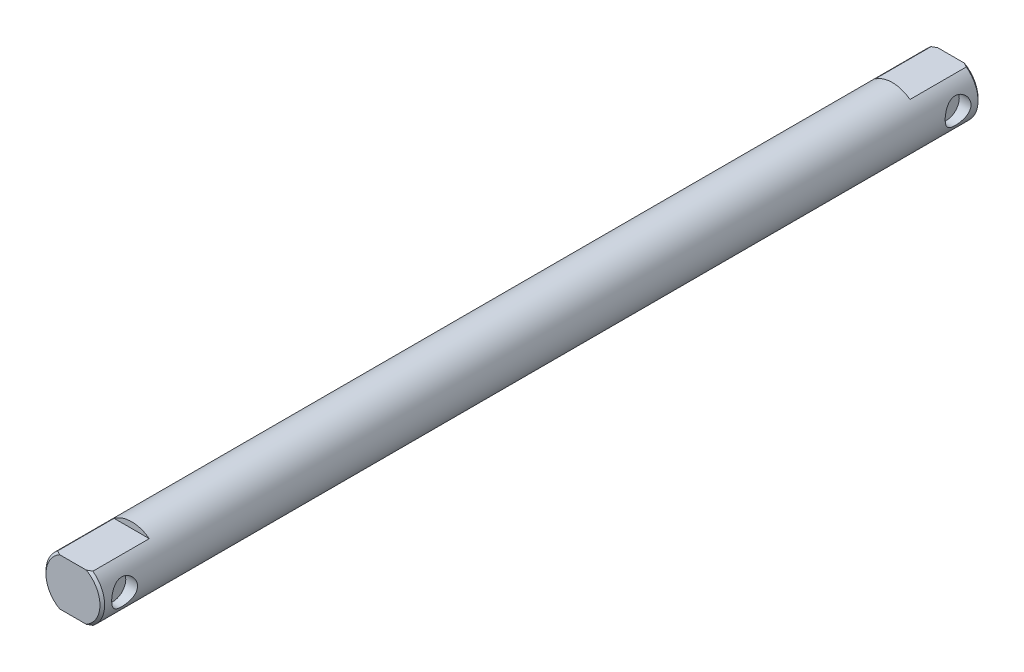
SolidWorks part; units mm, degrees
material "热轧圆钢 45"
ref_plane "前视基准面" through (0, 0, 0) normal (0, 0, 1) x (1, 0, 0)
ref_plane "上视基准面" through (0, 0, 0) normal (0, 1, 0) x (1, 0, 0)
ref_plane "右视基准面" through (0, 0, 0) normal (1, 0, 0) x (0, 0, -1)
sketch "草图1" plane through (0, 0, 0) normal (0, 0, 1) x (1, 0, 0)
  circle A0 centre (0, 0) radius 12.5
  dimension "D1" = 25
extrude "凸台-拉伸1" add sketch "草图1" along normal mid plane 374
chamfer "倒角1" distance 1 angle 45 2 edges at (12.5, 0, -187) (12.5, 0, 187)
ref_plane "基准面1" through (0, 12.5, 0) normal (0, 1, 0) x (1, 0, 0)
sketch "草图2" plane through (0, 12.5, 0) normal (0, 1, 0) x (1, 0, 0)
  line L0 (0, 0) -> (0, -174.5) construction
  line L1 (0, 0) -> (65.0447, 0) construction
  line L2 (-11.5, -187) -> (11.5, -187) construction
  line L3 (-12.5, -187) -> (12.5, -187)
  line L4 (-12.5, -187) -> (-12.5, -162)
  line L5 (-12.5, -162) -> (12.5, -162)
  line L6 (12.5, -187) -> (12.5, -162)
  line L7 (-12.5, -187) -> (12.5, -162) construction
  line L8 (-12.5, -162) -> (12.5, -187) construction
  line L9 (12.5, -186) -> (12.5, 186) construction
  line L10 (-12.5, 162) -> (12.5, 187) construction
  line L11 (-12.5, 187) -> (12.5, 162) construction
  line L12 (12.5, 187) -> (12.5, 162)
  line L13 (-12.5, 162) -> (12.5, 162)
  line L14 (-12.5, 187) -> (-12.5, 162)
  line L15 (-12.5, 187) -> (12.5, 187)
  dimension "D1" = 25
extrude "切除-拉伸1" cut sketch "草图2" against normal blind 2.5
mirror "镜向1" about plane through (0, 0, 0) normal (0, 1, 0) of "切除-拉伸1"
ref_plane "基准面2" through (12.5, 0, 0) normal (1, 0, 0) x (0, 0, -1)
sketch "草图3" plane through (12.5, 0, 0) normal (1, 0, 0) x (0, 0, -1)
  line L0 (-187, 0) -> (-177.5, 0) construction
  line L1 (-187, 10) -> (-187, -10) construction
  line L2 (-162, 12.5) -> (-162, 10) construction
  line L3 (0, 0) -> (0, 77.3708) construction
  circle A0 centre (-177.5, 0) radius 5.5
  circle A1 centre (177.5, 0) radius 5.5
  dimension "D2" = 11
  dimension "D1" = 15.5
extrude "切除-拉伸2" cut sketch "草图3" against normal blind 5
